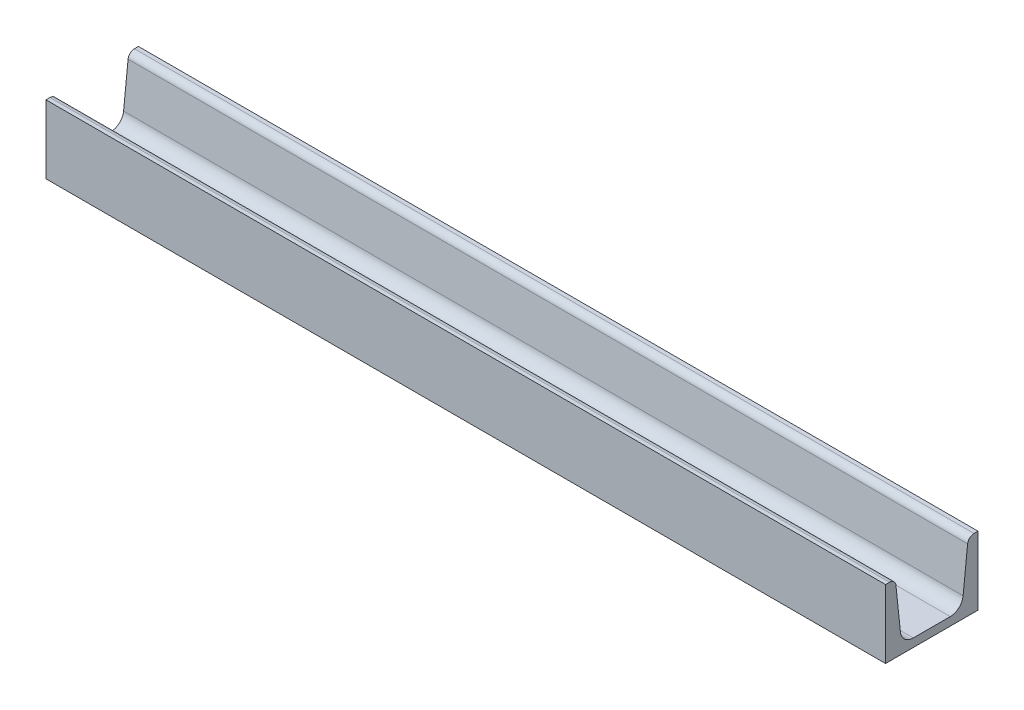
from build123d import *

# Parameters (mm, degrees)
GB_T_707_1988_HOT_ROLLED_CHANNEL_05_1_DEPTH = 454


with BuildPart() as part:
    # Sketch1 → GB/T 707-1988 hot-rolled channel 05(1) (new body)
    with BuildSketch(Plane.YZ.offset(-227)):
        with BuildLine():
            Line((37, 50), (0, 50))
            Line((0, 50), (0, 0))
            Line((0, 0), (37, 0))
            Line((37, 0), (37, 2.140642022))
            ThreePointArc((37, 2.140642022), (36.101006889, 4.482599144), (33.865849621, 5.621468656))
            Line((33.865849621, 5.621468656), (10.768300757, 8.049118866))
            ThreePointArc((10.768300757, 8.049118866), (6.297986222, 10.326857889), (4.5, 15.010772133))
            Line((4.5, 15.010772133), (4.5, 34.989227867))
            ThreePointArc((4.5, 34.989227867), (6.297986222, 39.673142111), (10.768300757, 41.950881134))
            Line((10.768300757, 41.950881134), (33.865849621, 44.378531344))
            ThreePointArc((33.865849621, 44.378531344), (36.101006889, 45.517400856), (37, 47.859357978))
            Line((37, 47.859357978), (37, 50))
        make_face()
    extrude(amount=GB_T_707_1988_HOT_ROLLED_CHANNEL_05_1_DEPTH)


solid = part.part
